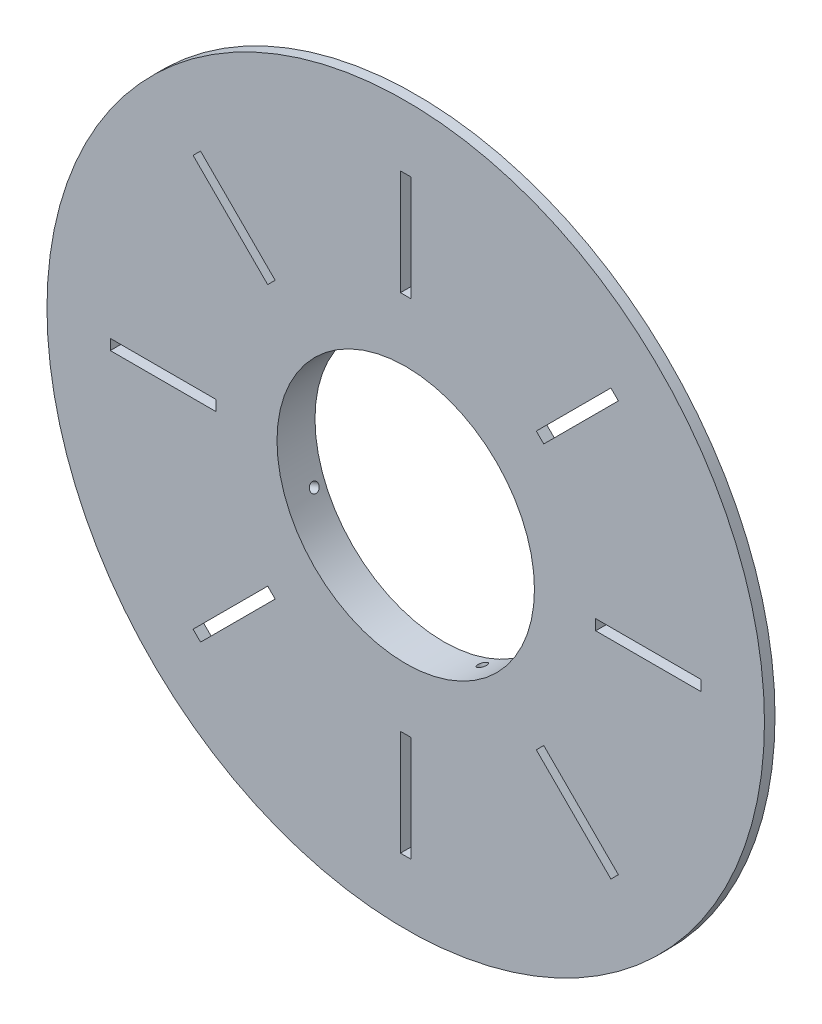
SolidWorks part; units mm, degrees
ref_plane "前视基准面" through (0, 0, 0) normal (0, 0, 1) x (1, 0, 0)
ref_plane "上视基准面" through (0, 0, 0) normal (0, 1, 0) x (1, 0, 0)
ref_plane "右视基准面" through (0, 0, 0) normal (1, 0, 0) x (0, 0, -1)
sketch "草图1" plane through (0, 0, 0) normal (0, 0, 1) x (1, 0, 0)
  circle A0 centre (0, 0) radius 170
  circle A1 centre (0, 0) radius 61
  dimension "D1" = 340
  dimension "D2" = 122
extrude "凸台-拉伸1" add sketch "草图1" along normal mid plane 5
sketch "草图2" plane through (0, 0, -2.5) normal (0, 0, -1) x (-1, 0, 0)
  line L0 (0, 0) -> (0, 90) construction
  line L1 (2.5, 90) -> (-2.5, 90)
  line L2 (2.5, 90) -> (2.5, 140)
  line L3 (2.5, 140) -> (-2.5, 140)
  line L4 (-2.5, 90) -> (-2.5, 140)
  line L5 (2.5, 90) -> (-2.5, 140) construction
  line L6 (2.5, 140) -> (-2.5, 90) construction
  point P0 (0, 115)
  dimension "D1" = 90
  dimension "D2" = 50
  dimension "D3" = 5
extrude "切除-拉伸1" cut sketch "草图2" against normal blind 606
pattern_circular "阵列(圆周)1" count 8 over 360 about axis through (0, 0, 0) along (0, 0, 1) of "切除-拉伸1"
sketch "草图3" plane through (0, 0, -2.5) normal (0, 0, -1) x (-1, 0, 0)
  circle A0 centre (0, 0) radius 61 construction
  circle A1 centre (0, 0) radius 61
  circle A2 centre (0, 0) radius 71
  dimension "D1" = 10
extrude "凸台-拉伸2" add sketch "草图3" along normal blind 13
ref_plane "基准面1" through (0, 0, -10.5) normal (0, 0, -1) x (-1, 0, 0)
sketch "草图4" plane through (0, 0, -10.5) normal (0, 0, -1) x (-1, 0, 0)
  line L0 (0, 0) -> (42.278, 102.0682) construction
  line L1 (2.5, 90) -> (2.5, 140) construction
  line L2 (32.9591, 79.5703) -> (34.9916, 78.7284)
  line L3 (34.9916, 78.7284) -> (19.1953, 40.5927)
  line L4 (19.1953, 40.5927) -> (17.1628, 41.4346)
  line L5 (17.1628, 41.4346) -> (33.3167, 80.4337)
  dimension "D1" = 22.5
  dimension "D2" = 2.2
revolve "切除-旋转1" cut sketch "草图4" angle 360 about L0
pattern_circular "阵列(圆周)2" count 4 over 360 about axis through (0, 0, 2.5) along (0, 0, -1) of "切除-旋转1"
